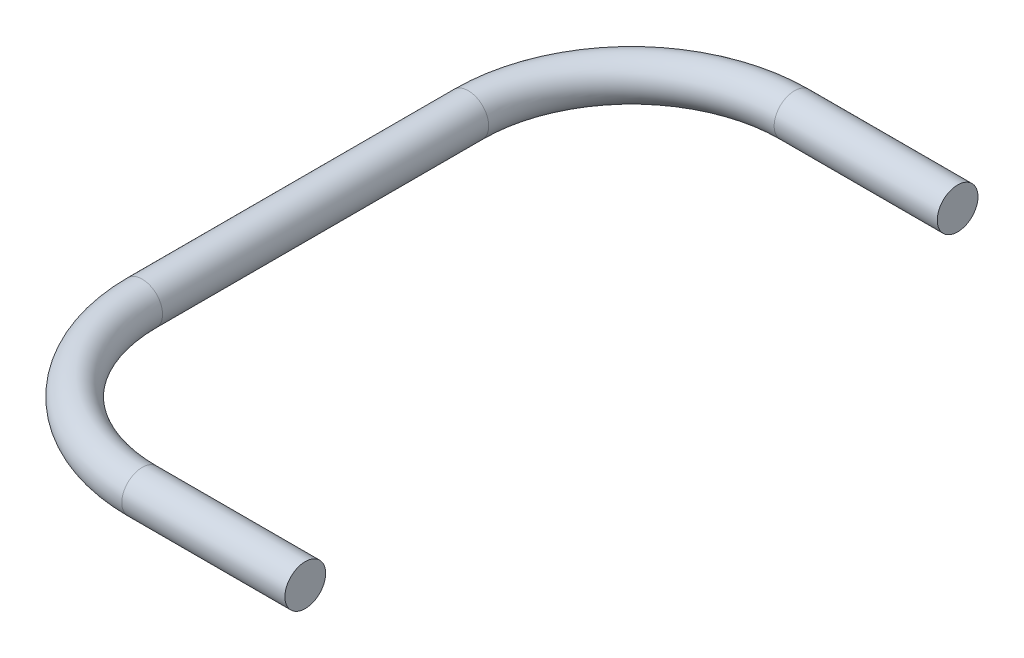
from build123d import *

# Parameters (mm, degrees)
SKETCH2_R = 2.5


with BuildPart() as part:
    # Sweep1: sweep along a path in Sketch1
    with BuildLine(Plane(origin=(0, 0, 0), x_dir=(1, 0, 0), z_dir=(0, 1, 0))) as sweep1_path:
        Line((0, 0), (-20, 0))
        ThreePointArc((-20, 0), (-34.142135624, -5.857864376), (-40, -20))
        Line((-40, -20), (-40, -60))
        ThreePointArc((-40, -60), (-34.142135624, -74.142135624), (-20, -80))
        Line((-20, -80), (0, -80))
    # Sketch2 → Sweep1 (sweep)
    with BuildSketch(Plane(origin=(0, 0, 0), x_dir=(0, 0, -1), z_dir=(1, 0, 0))):
        Circle(SKETCH2_R)
    sweep(path=sweep1_path.line)


solid = part.part
